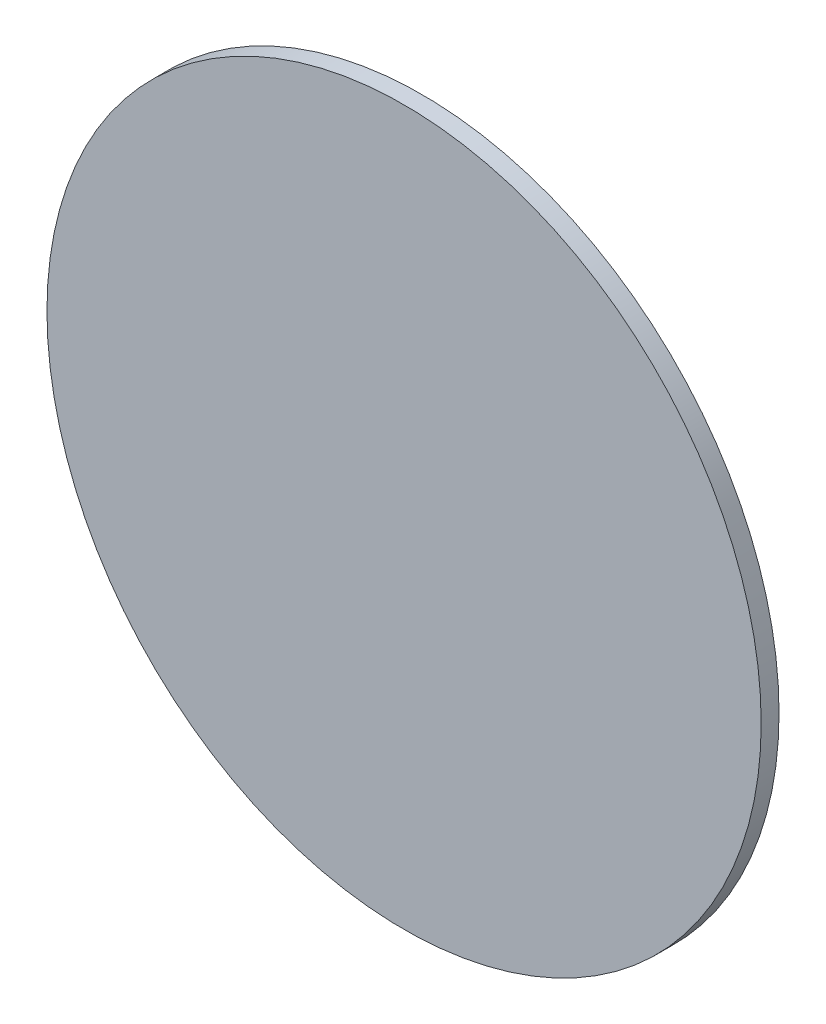
from build123d import *

# Parameters (mm, degrees)
SKETCH1_R           = 20
BOSS_EXTRUDE1_DEPTH = 1
SKETCH2_R           = 2
BOSS_EXTRUDE2_DEPTH = 1
SKETCH3_R           = 12.5
BOSS_EXTRUDE3_DEPTH = 1


with BuildPart() as part:
    # Sketch1 → Boss-Extrude1 (new body)
    with BuildSketch(Plane.XY):
        Circle(SKETCH1_R)
    extrude(amount=BOSS_EXTRUDE1_DEPTH)

    # Sketch2 → Boss-Extrude2 (add)
    with BuildSketch(Plane(origin=(0, 0, 0), x_dir=(-1, 0, 0), z_dir=(0, 0, -1))):
        with Locations(Location((0, 0, 0), (0, 0, 180))):
            Circle(SKETCH2_R)
    extrude(amount=BOSS_EXTRUDE2_DEPTH)

    # Sketch3 → Boss-Extrude3 (add)
    with BuildSketch(Plane(origin=(0, 0, -1), x_dir=(-1, 0, 0), z_dir=(0, 0, -1))):
        Circle(SKETCH3_R)
    extrude(amount=BOSS_EXTRUDE3_DEPTH)


solid = part.part
